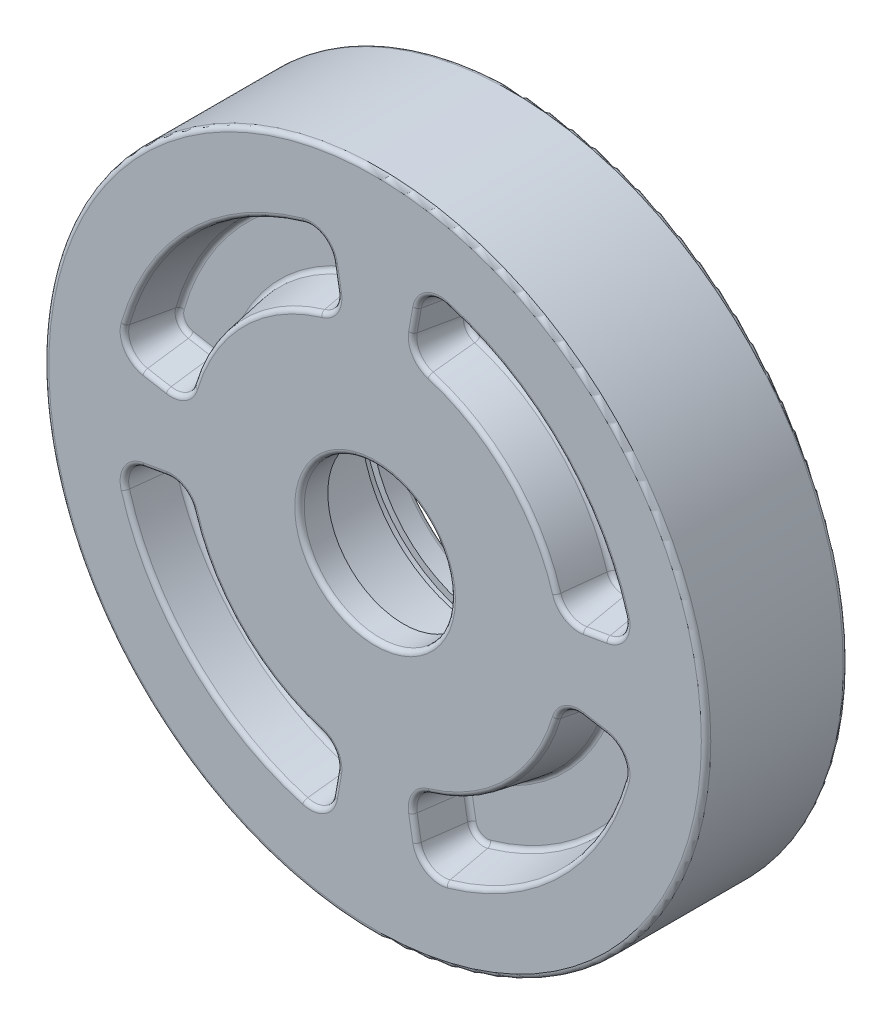
SolidWorks part; units mm, degrees
ref_plane "Front Plane" through (0, 0, 0) normal (0, 0, 1) x (1, 0, 0)
ref_plane "Top Plane" through (0, 0, 0) normal (0, 1, 0) x (1, 0, 0)
ref_plane "Right Plane" through (0, 0, 0) normal (1, 0, 0) x (0, 0, -1)
sketch "Sketch1" plane through (0, 0, 0) normal (0, 0, 1) x (1, 0, 0)
  circle A0 centre (0, 0) radius 70
  dimension "D1" = 140
extrude "Boss-Extrude1" add sketch "Sketch1" along normal mid plane 30
sketch "Sketch2" plane through (0, 0, 15) normal (0, 0, 1) x (1, 0, 0)
  circle A0 centre (0, 0) radius 16
  dimension "D1" = 32
extrude "Cut-Extrude1" cut sketch "Sketch2" against normal blind 6
sketch "Sketch3" plane through (0, 0, 9) normal (0, 0, 1) x (1, 0, 0)
  circle A0 centre (0, 0) radius 22.5
  dimension "D1" = 45
extrude "Cut-Extrude2" cut sketch "Sketch3" against normal blind 2
sketch "Sketch4" plane through (0, 0, 7) normal (0, 0, 1) x (1, 0, 0)
  circle A0 centre (0, 0) radius 26
  dimension "D1" = 52
extrude "Cut-Extrude3" cut sketch "Sketch4" against normal blind 15
sketch "Sketch5" plane through (0, 0, -8) normal (0, 0, 1) x (1, 0, 0)
  circle A0 centre (0, 0) radius 27.5
  dimension "D1" = 55
extrude "Cut-Extrude4" cut sketch "Sketch5" against normal blind 2
sketch "Sketch6" plane through (0, 0, -10) normal (0, 0, 1) x (1, 0, 0)
  circle A0 centre (0, 0) radius 26
  dimension "D1" = 52
extrude "Cut-Extrude5" cut sketch "Sketch6" against normal through all
sketch "Sketch7" plane through (0, 0, -15) normal (0, 0, -1) x (-1, 0, 0)
  line L1 (-8.8005, 48.9423) -> (-7.9322, 43.9872)
  line L7 (-48.9423, 8.8005) -> (-43.9872, 7.9322)
  arc A0 (-11.4286, 38.3326) -> (-38.3326, 11.4286) centre (0, 0) ccw
  arc A1 (-15.098, 52.8871) -> (-52.8871, 15.098) centre (0, 0) ccw
  arc A2 (-11.4286, 38.3326) -> (-7.9322, 43.9872) centre (-12.8571, 43.1242) ccw
  arc A3 (-15.098, 52.8871) -> (-8.8005, 48.9423) centre (-13.7255, 48.0792) cw
  arc A4 (-38.3326, 11.4286) -> (-43.9872, 7.9322) centre (-43.1242, 12.8571) cw
  arc A5 (-48.9423, 8.8005) -> (-52.8871, 15.098) centre (-48.0792, 13.7255) cw
  point P4 (0, 60.3583)
  point P5 (0, 33.3418)
  point P24 (0, 0)
  dimension "D1" = 80
  dimension "D2" = 110
  dimension "D3" = 5
  dimension "D4" = 5
extrude "Cut-Extrude6" cut sketch "Sketch7" against normal blind 10 draft 10
pattern_circular "CirPattern1" count 4 over 360 about axis through (0, 0, 0) along (0, 0, 1) of "Cut-Extrude6"
mirror "Mirror1" about plane through (0, 0, 0) normal (0, 0, 1) of "CirPattern1", "Cut-Extrude6"
fillet "Fillet1" radius 1 66 edges at (29.5311, -29.5311, -5) (10.1042, -41.422, -5) (10.1032, -46.1604, -5) (12.0072, -50.8222, -5) (37.6441, -37.6441, -5) (50.8222, -12.0072, -5) (46.1604, -10.1032, -5) (41.422, -10.1042, -5) (-29.5311, -29.5311, -5) (-41.422, -10.1042, -5) (-46.1604, -10.1032, -5) (-50.8222, -12.0072, -5) (-37.6441, -37.6441, -5) (-12.0072, -50.8222, -5) (-10.1032, -46.1604, -5) (-10.1042, -41.422, -5) (29.5311, 29.5311, -5) (41.422, 10.1042, -5) (46.1604, 10.1032, -5) (50.8222, 12.0072, -5) (37.6441, 37.6441, -5) (12.0072, 50.8222, -5) (10.1032, 46.1604, -5) (10.1042, 41.422, -5) (-29.5311, 29.5311, -5) (-10.1042, 41.422, -5) (-10.1032, 46.1604, -5) (-12.0072, 50.8222, -5) (-37.6441, 37.6441, -5) (-50.8222, 12.0072, -5) (-46.1604, 10.1032, -5) (-41.422, 10.1042, -5) (70, 0, -15) (26, 0, -15) (11.0712, 52.3165, -15) (38.8909, 38.8909, -15) (52.3165, 11.0712, -15) (46.4648, 8.3664, -15) (40.4946, 8.6044, -15) (28.2843, 28.2843, -15) (8.6044, 40.4946, -15) (8.3664, 46.4648, -15) (52.3165, -11.0712, -15) (38.8909, -38.8909, -15) (11.0712, -52.3165, -15) (8.3664, -46.4648, -15) (8.6044, -40.4946, -15) (28.2843, -28.2843, -15) (40.4946, -8.6044, -15) (46.4648, -8.3664, -15) (-11.0712, -52.3165, -15) (-38.8909, -38.8909, -15) (-52.3165, -11.0712, -15) (-46.4648, -8.3664, -15) (-40.4946, -8.6044, -15) (-28.2843, -28.2843, -15) (-8.6044, -40.4946, -15) (-8.3664, -46.4648, -15) (-52.3165, 11.0712, -15) (-38.8909, 38.8909, -15) (-11.0712, 52.3165, -15) (-8.3664, 46.4648, -15) (-8.6044, 40.4946, -15) (-28.2843, 28.2843, -15) (-40.4946, 8.6044, -15) (-46.4648, 8.3664, -15)
fillet "Fillet2" radius 1 66 edges at (-8.6044, 40.4946, 15) (-8.3664, 46.4648, 15) (-11.0712, 52.3165, 15) (-38.8909, 38.8909, 15) (-52.3165, 11.0712, 15) (-46.4648, 8.3664, 15) (-40.4946, 8.6044, 15) (-28.2843, 28.2843, 15) (8.6044, -40.4946, 15) (8.3664, -46.4648, 15) (11.0712, -52.3165, 15) (38.8909, -38.8909, 15) (52.3165, -11.0712, 15) (46.4648, -8.3664, 15) (40.4946, -8.6044, 15) (28.2843, -28.2843, 15) (70, 0, 15) (16, 0, 15) (40.4946, 8.6044, 15) (46.4648, 8.3664, 15) (52.3165, 11.0712, 15) (38.8909, 38.8909, 15) (11.0712, 52.3165, 15) (8.3664, 46.4648, 15) (8.6044, 40.4946, 15) (28.2843, 28.2843, 15) (-40.4946, -8.6044, 15) (-46.4648, -8.3664, 15) (-52.3165, -11.0712, 15) (-38.8909, -38.8909, 15) (-11.0712, -52.3165, 15) (-8.3664, -46.4648, 15) (-8.6044, -40.4946, 15) (-28.2843, -28.2843, 15) (-10.1032, -46.1604, 5) (-12.0072, -50.8222, 5) (-37.6441, -37.6441, 5) (-50.8222, -12.0072, 5) (-46.1604, -10.1032, 5) (-41.422, -10.1042, 5) (-29.5311, -29.5311, 5) (-10.1042, -41.422, 5) (46.1604, -10.1032, 5) (50.8222, -12.0072, 5) (37.6441, -37.6441, 5) (12.0072, -50.8222, 5) (10.1032, -46.1604, 5) (10.1042, -41.422, 5) (29.5311, -29.5311, 5) (41.422, -10.1042, 5) (10.1032, 46.1604, 5) (12.0072, 50.8222, 5) (37.6441, 37.6441, 5) (50.8222, 12.0072, 5) (46.1604, 10.1032, 5) (41.422, 10.1042, 5) (29.5311, 29.5311, 5) (10.1042, 41.422, 5) (-46.1604, 10.1032, 5) (-50.8222, 12.0072, 5) (-37.6441, 37.6441, 5) (-12.0072, 50.8222, 5) (-10.1032, 46.1604, 5) (-10.1042, 41.422, 5) (-29.5311, 29.5311, 5) (-41.422, 10.1042, 5)
sketch "Sketch8" plane through (0, 0, -15) normal (0, 0, -1) x (-1, 0, 0)
  circle A1 centre (0, 32.5) radius 1.5
  circle A2 centre (28.1458, -16.25) radius 1.5
  circle A3 centre (-28.1458, -16.25) radius 1.5
  point P12 (0, 0)
  dimension "D2" = 3
  dimension "D3" = 3
extrude "Cut-Extrude7" cut sketch "Sketch8" against normal blind 10
